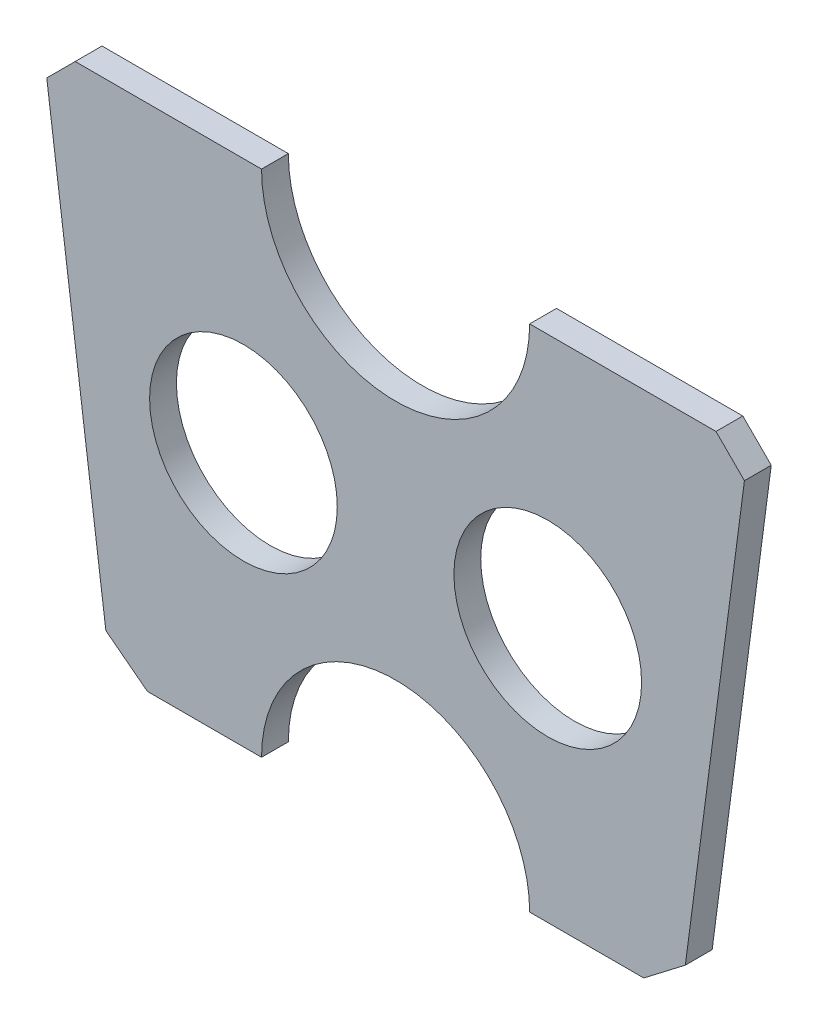
from build123d import *

# Parameters (mm, degrees)
SKETCH1_R           = 35
BOSS_EXTRUDE1_DEPTH = 10


with BuildPart() as part:
    # Sketch1 → Boss-Extrude1 (new body)
    with BuildSketch(Plane.XY):
        with BuildLine():
            Line((50, 95), (119.5, 95))
            Line((119.5, 95), (130.104651163, 84.395348837))
            Line((130.104651163, 84.395348837), (108.065454151, -83.102548453))
            Line((108.065454151, -83.102548453), (92.562714257, -95))
            Line((92.562714257, -95), (50, -95))
            ThreePointArc((50, -95), (0, -45), (-50, -95))
            Line((-50, -95), (-92.562714257, -95))
            Line((-92.562714257, -95), (-108.065454151, -83.102548453))
            Line((-108.065454151, -83.102548453), (-130.104651163, 84.395348837))
            Line((-130.104651163, 84.395348837), (-119.5, 95))
            Line((-119.5, 95), (-50, 95))
            ThreePointArc((-50, 95), (0, 45), (50, 95))
        make_face()
        with Locations((56.75, 0)):
            Circle(SKETCH1_R, mode=Mode.SUBTRACT)
        with Locations(Location((-56.75, 0, 0), (0, 0, 180))):
            Circle(SKETCH1_R, mode=Mode.SUBTRACT)
    extrude(amount=BOSS_EXTRUDE1_DEPTH)


solid = part.part
